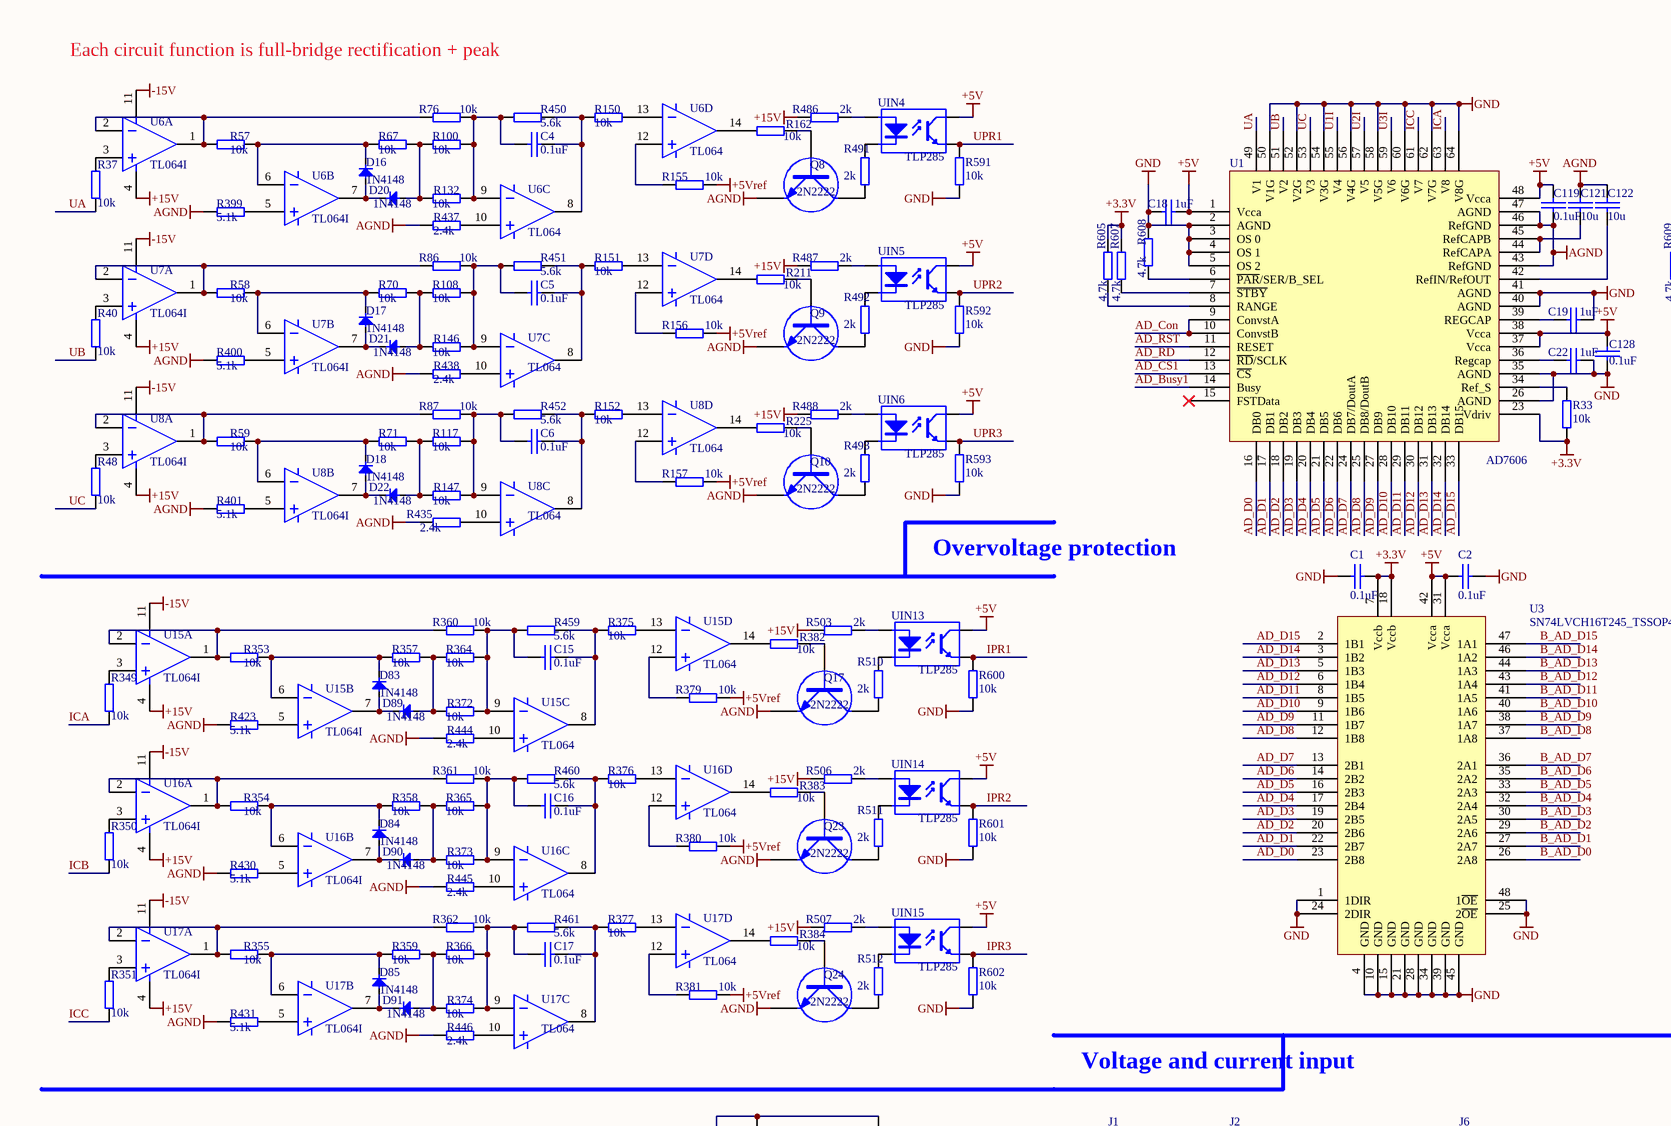
[diagram p0: MISC80584.SchDoc, top left]
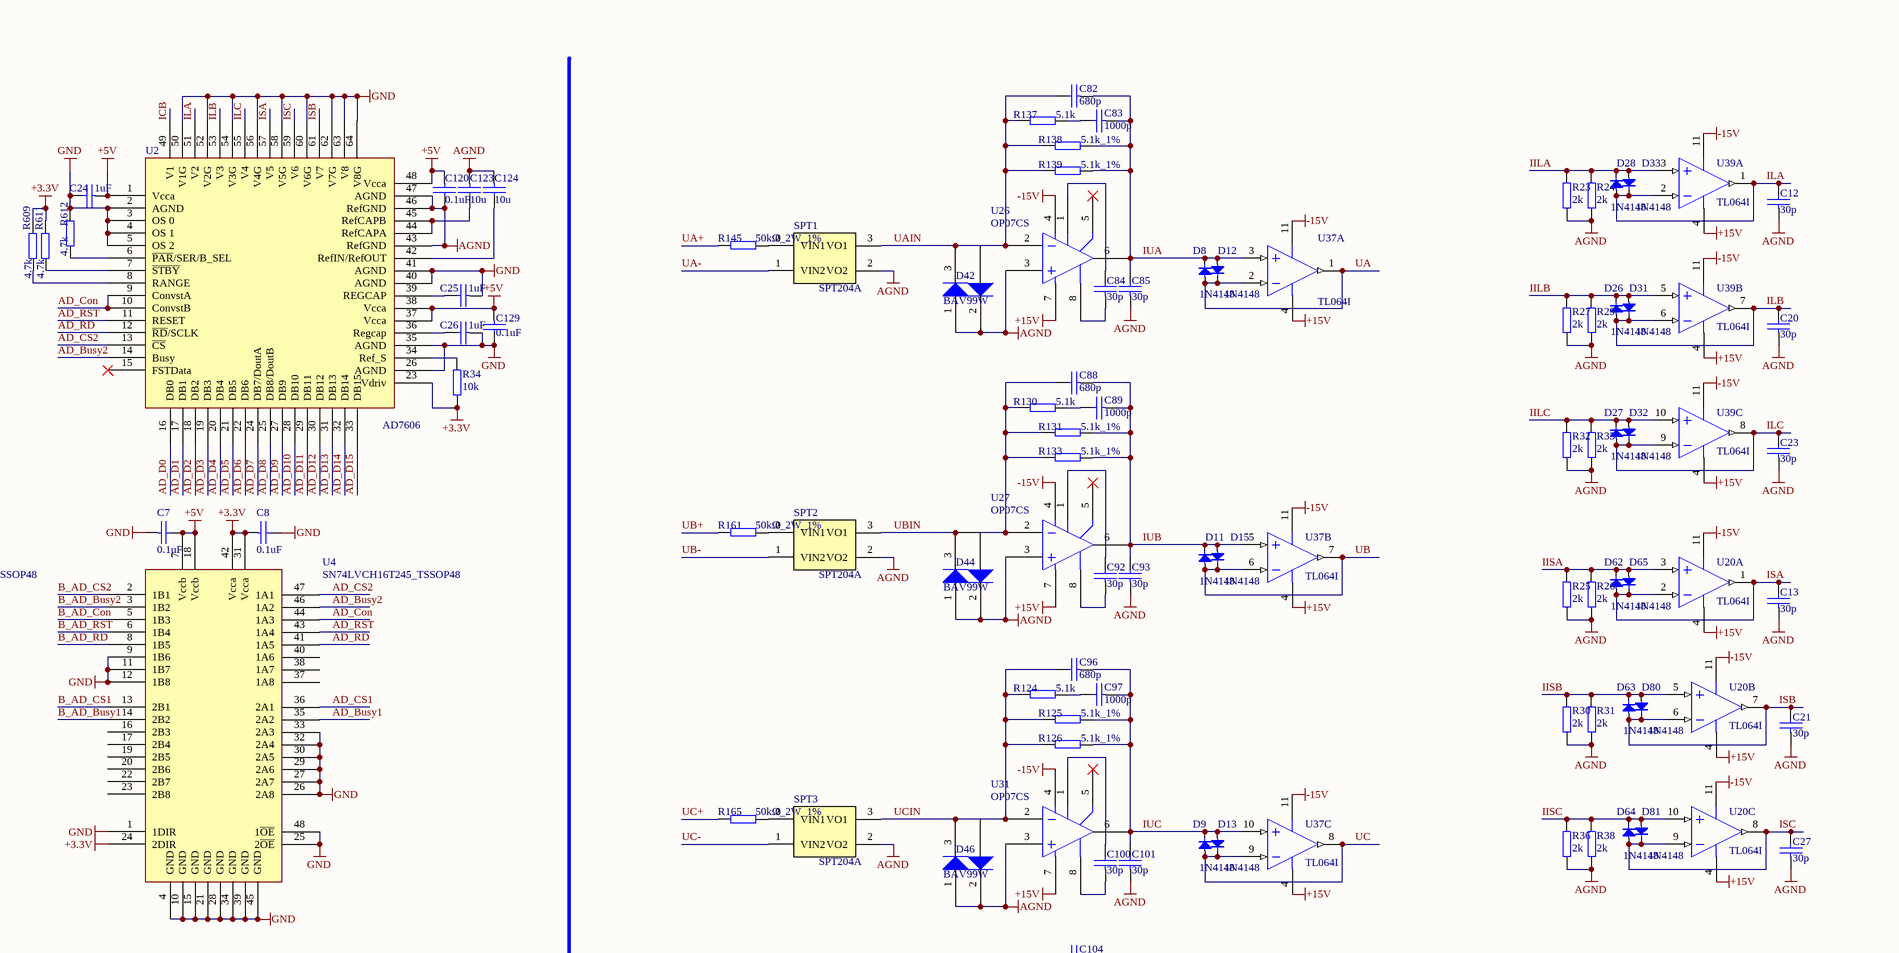
[diagram p1: MISC80584.SchDoc, top right]
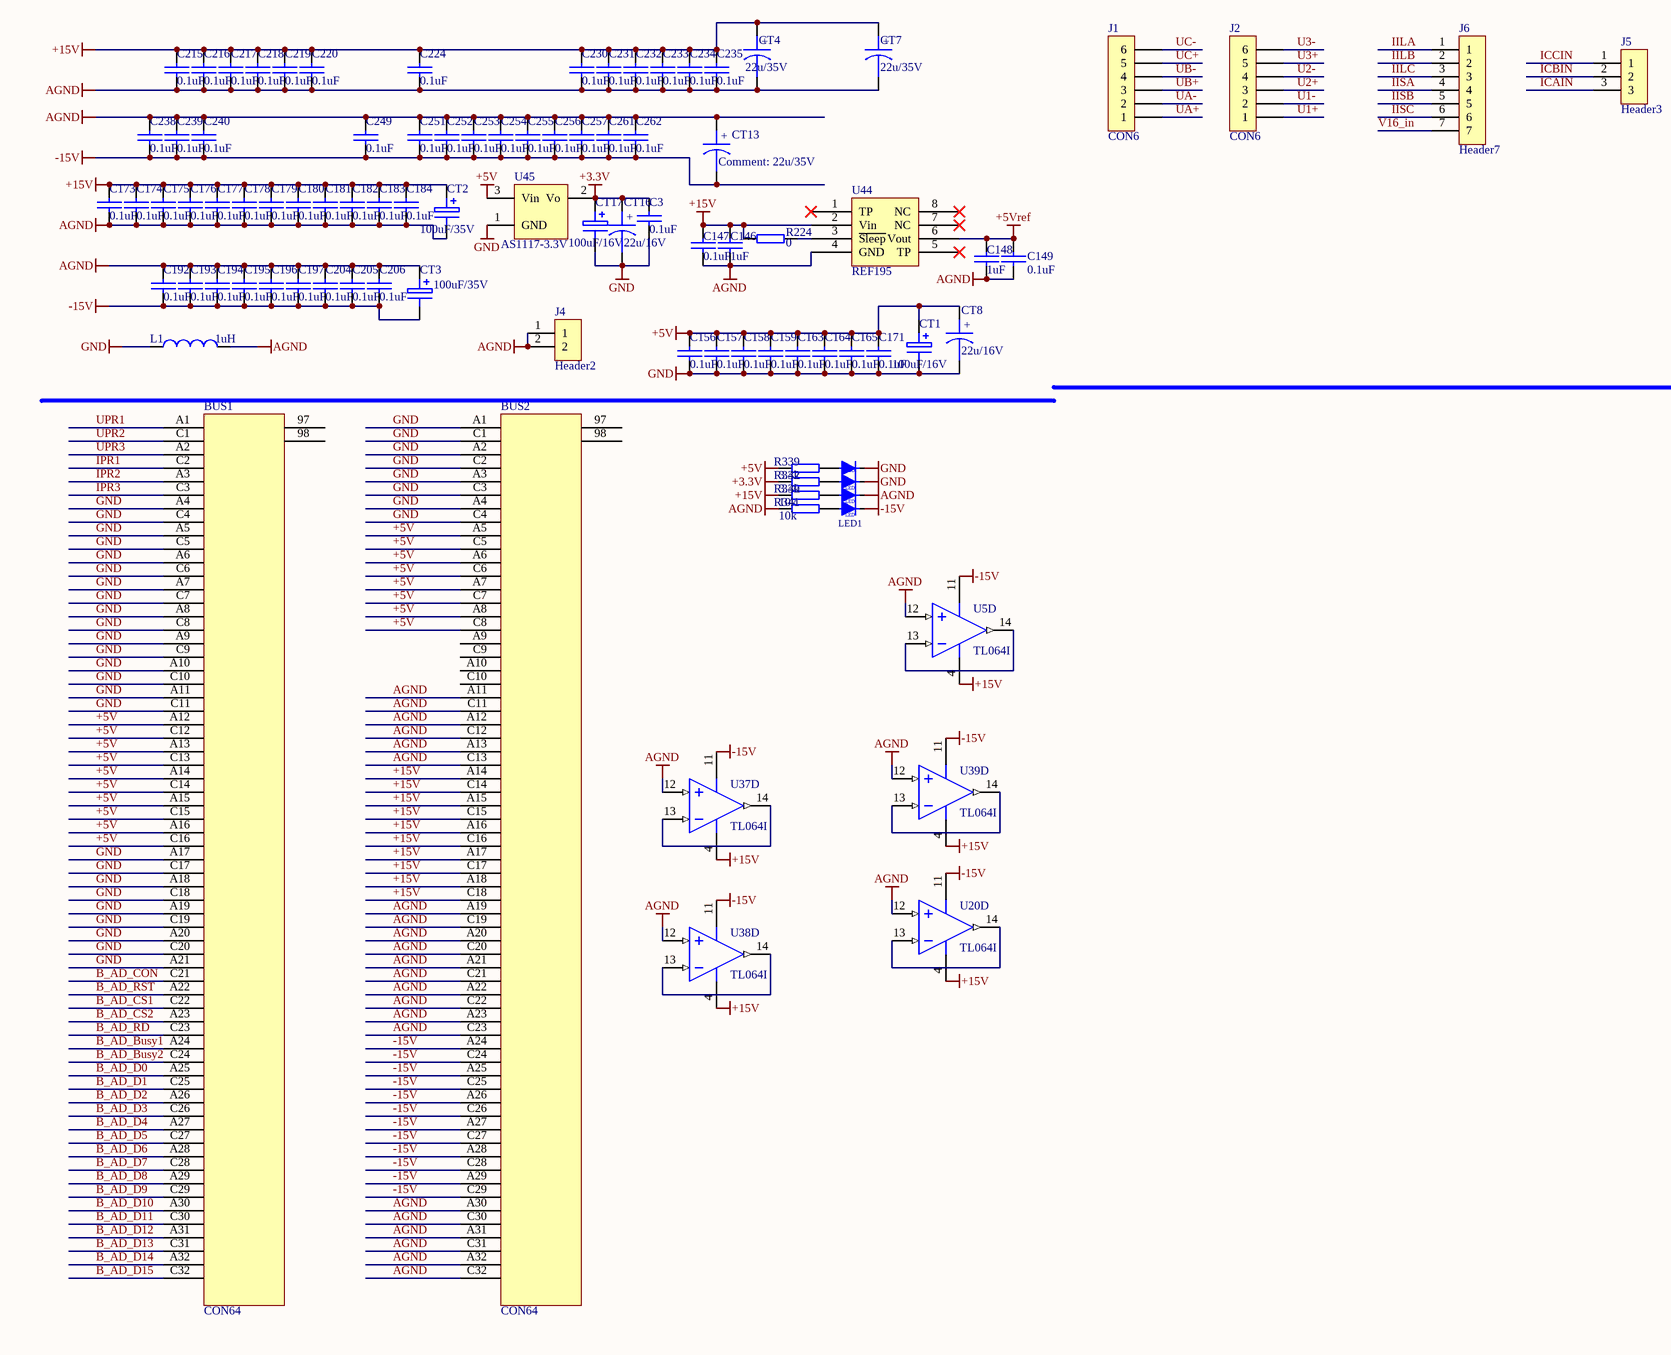
[diagram p2: MISC80584.SchDoc, bottom left]
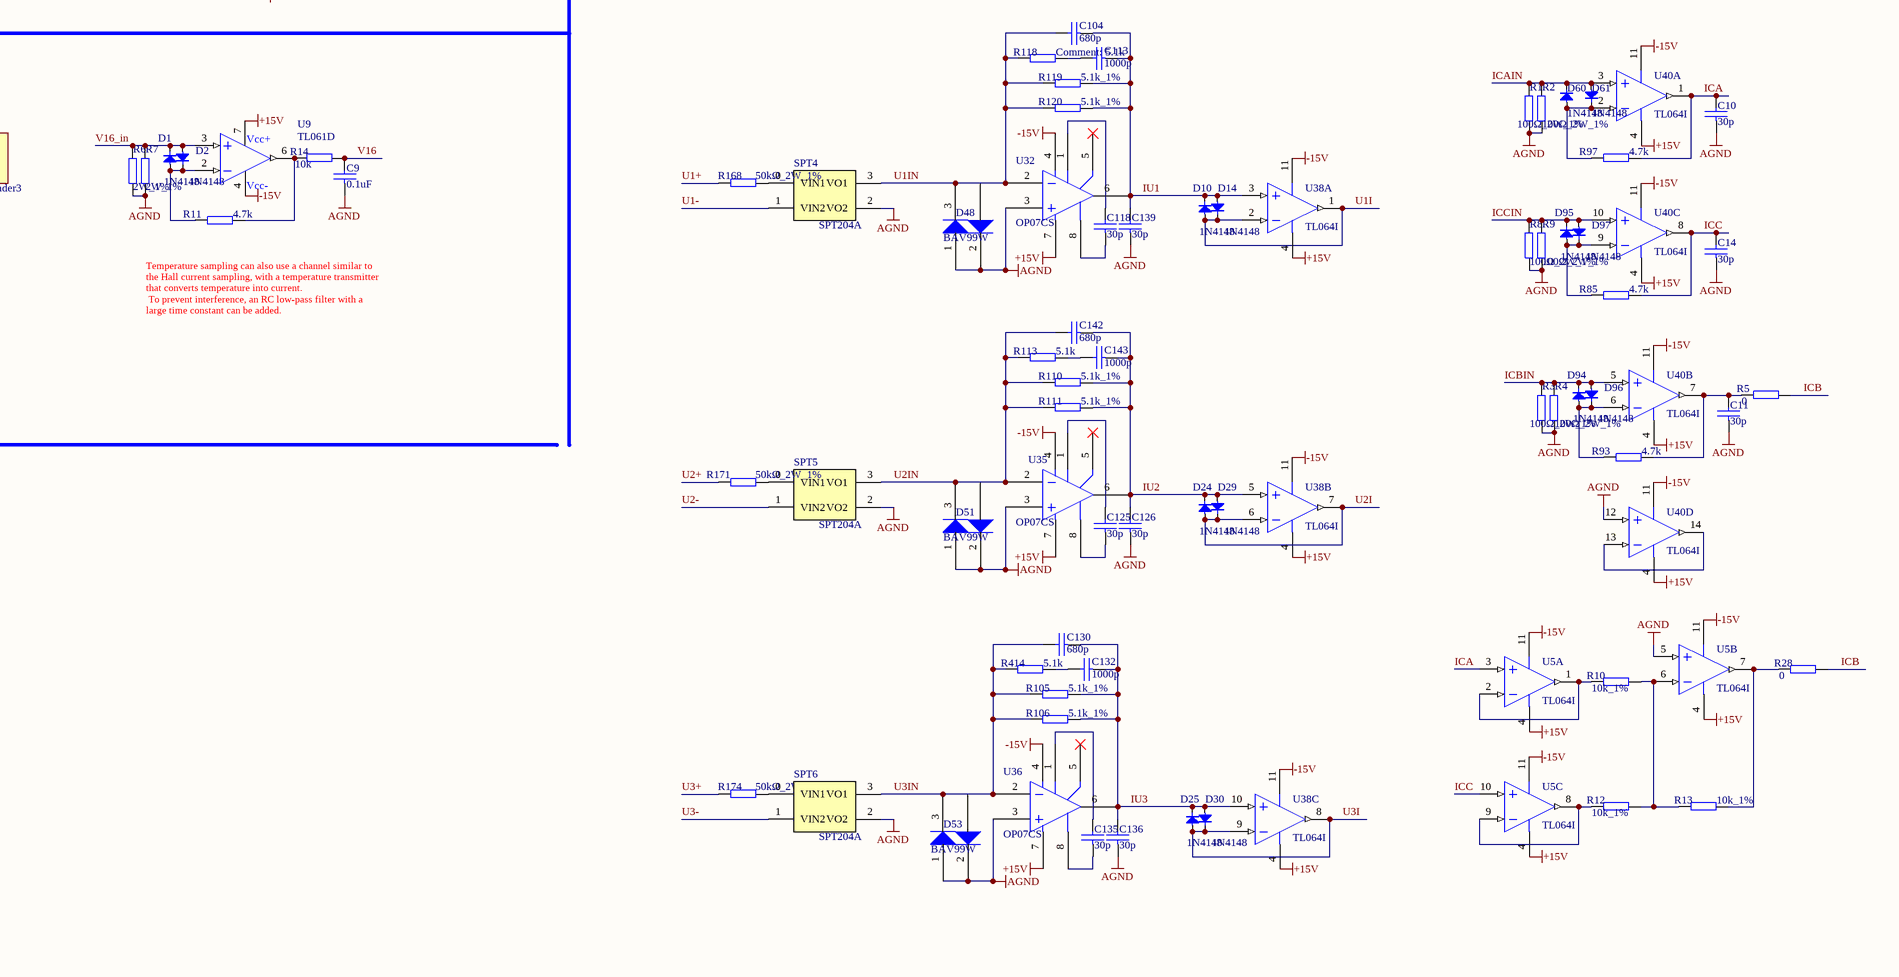
[diagram p3: MISC80584.SchDoc, bottom right]
# Altium project MISC80584.PrjPCB
1 sheet, 386 parts. Net scope: global (net labels, ports and power ports of the same name join across sheets).
Board file: MISC80584.PCBDoc

## Sheet MISC80584.SchDoc
size 762 x 457 mm; SheetNumber: 0; SheetTotal: 0

### Parts
BUS1  CON64  [BUS64W-A]
BUS2  CON64  [BUS64W-A]
C1  0.1uF  [0603]
C2  0.1uF  [0603]
C3  0.1uF  [0603]
C4  0.1uF  [0603]
C5  0.1uF  [0603]
C6  0.1uF  [0603]
C7  0.1uF  [0603]
C8  0.1uF  [0603]
C9  0.1uF  [0603]
C10  30p  [0603]
C11  30p  [0603]
C12  30p  [0603]
C13  30p  [0603]
C14  30p  [0603]
C15  0.1uF  [0603]
C16  0.1uF  [0603]
C17  0.1uF  [0603]
C18  1uF  [0603]
C19  1uF  [0603]
C20  30p  [0603]
C21  30p  [0603]
C22  1uF  [0603]
C23  30p  [0603]
C24  1uF  [0603]
C25  1uF  [0603]
C26  1uF  [0603]
C27  30p  [0603]
C82  680p  [0603]
C83  1000p  [0603]
C84  30p  [0603]
C85  30p  [0603]
C88  680p  [0603]
C89  1000p  [0603]
C92  30p  [0603]
C93  30p  [0603]
C96  680p  [0603]
C97  1000p  [0603]
C100  30p  [0603]
C101  30p  [0603]
C104  680p  [0603]
C113  1000p  [0603]
C118  30p  [0603]
C119  0.1uF  [0603]
C120  0.1uF  [0603]
C121  10u  [0805]
C122  10u  [0805]
C123  10u  [0805]
C124  10u  [0805]
C125  30p  [0603]
C126  30p  [0603]
C128  0.1uF  [0603]
C129  0.1uF  [0603]
C130  680p  [0603]
C132  1000p  [0603]
C135  30p  [0603]
C136  30p  [0603]
C139  30p  [0603]
C142  680p  [0603]
C143  1000p  [0603]
C146  1uF  [0603]
C147  0.1uF  [0603]
C148  1uF  [0603]
C149  0.1uF  [0603]
C156  0.1uF  [0603]
C157  0.1uF  [0603]
C158  0.1uF  [0603]
C159  0.1uF  [0603]
C163  0.1uF  [0603]
C164  0.1uF  [0603]
C165  0.1uF  [0603]
C171  0.1uF  [0603]
C173  0.1uF  [0603]
C174  0.1uF  [0603]
C175  0.1uF  [0603]
C176  0.1uF  [0603]
C177  0.1uF  [0603]
C178  0.1uF  [0603]
C179  0.1uF  [0603]
C180  0.1uF  [0603]
C181  0.1uF  [0603]
C182  0.1uF  [0603]
C183  0.1uF  [0603]
C184  0.1uF  [0603]
C192  0.1uF  [0603]
C193  0.1uF  [0603]
C194  0.1uF  [0603]
C195  0.1uF  [0603]
C196  0.1uF  [0603]
C197  0.1uF  [0603]
C204  0.1uF  [0603]
C205  0.1uF  [0603]
C206  0.1uF  [0603]
C215  0.1uF  [0603]
C216  0.1uF  [0603]
C217  0.1uF  [0603]
C218  0.1uF  [0603]
C219  0.1uF  [0603]
C220  0.1uF  [0603]
C224  0.1uF  [0603]
C230  0.1uF  [0603]
C231  0.1uF  [0603]
C232  0.1uF  [0603]
C233  0.1uF  [0603]
C234  0.1uF  [0603]
C235  0.1uF  [0603]
C238  0.1uF  [0603]
C239  0.1uF  [0603]
C240  0.1uF  [0603]
C249  0.1uF  [0603]
C251  0.1uF  [0603]
C252  0.1uF  [0603]
C253  0.1uF  [0603]
C254  0.1uF  [0603]
C255  0.1uF  [0603]
C256  0.1uF  [0603]
C257  0.1uF  [0603]
C261  0.1uF  [0603]
C262  0.1uF  [0603]
CT1  100uF/16V  [L470UF]
CT2  100uF/35V  [L470UF]
CT3  100uF/35V  [L470UF]
CT4  22u/35V  [7343_CASE-D]
CT7  22u/35V  [7343_CASE-D]
CT8  22u/16V  [3528_CASE-B]
CT13  22u/35V  [7343_CASE-D]
CT16  22u/16V  [3528_CASE-B]
CT17  100uF/16V  [L470UF]
D1  1N4148  [1N4148-A]
D2  1N4148  [1N4148-A]
D8  1N4148  [1N4148-A]
D9  1N4148  [1N4148-A]
D10  1N4148  [1N4148-A]
D11  1N4148  [1N4148-A]
D12  1N4148  [1N4148-A]
D13  1N4148  [1N4148-A]
D14  1N4148  [1N4148-A]
D15  1N4148  [1N4148-A]
D16  1N4148  [1N4148-A]
D17  1N4148  [1N4148-A]
D18  1N4148  [1N4148-A]
D20  1N4148  [1N4148-A]
D21  1N4148  [1N4148-A]
D22  1N4148  [1N4148-A]
D24  1N4148  [1N4148-A]
D25  1N4148  [1N4148-A]
D26  1N4148  [1N4148-A]
D27  1N4148  [1N4148-A]
D28  1N4148  [1N4148-A]
D29  1N4148  [1N4148-A]
D30  1N4148  [1N4148-A]
D31  1N4148  [1N4148-A]
D32  1N4148  [1N4148-A]
D33  1N4148  [1N4148-A]
D42  BAV99W  [SOT23R]
D44  BAV99W  [SOT23R]
D46  BAV99W  [SOT23R]
D48  BAV99W  [SOT23R]
D51  BAV99W  [SOT23R]
D53  BAV99W  [SOT23R]
D60  1N4148  [1N4148-A]
D61  1N4148  [1N4148-A]
D62  1N4148  [1N4148-A]
D63  1N4148  [1N4148-A]
D64  1N4148  [1N4148-A]
D65  1N4148  [1N4148-A]
D80  1N4148  [1N4148-A]
D81  1N4148  [1N4148-A]
D83  1N4148  [1N4148-A]
D84  1N4148  [1N4148-A]
D85  1N4148  [1N4148-A]
D89  1N4148  [1N4148-A]
D90  1N4148  [1N4148-A]
D91  1N4148  [1N4148-A]
D94  1N4148  [1N4148-A]
D95  1N4148  [1N4148-A]
D96  1N4148  [1N4148-A]
D97  1N4148  [1N4148-A]
J1  CON6  [EDGCon_6P_5.08mm_ear]
J2  CON6  [EDGCon_6P_5.08mm_ear]
J4  Header2  [EDGCON_2p_5.08mm_ear]
J5  Header3  [EDGCON_3p_5.08mm_ear]
J6  Header7  [EDGCon_7P_5.08mm_ear]
L1  1uH  [0805]
LED1  LEDGroup_4  [LEDGroup_4]  (value not drawn)
Q8  2N2222  [SOT23-3]
Q9  2N2222  [SOT23-3]
Q10  2N2222  [SOT23-3]
Q17  2N2222  [SOT23-3]
Q23  2N2222  [SOT23-3]
Q24  2N2222  [SOT23-3]
R1  100Ω_2W_1%  [AXIAL0.8]
R2  100Ω_2W_1%  [AXIAL0.8]
R3  100Ω_2W_1%  [AXIAL0.8]
R4  100Ω_2W_1%  [AXIAL0.8]
R5  0  [0603]
R6  2W_1%  [AXIAL0.8]
R7  2W_1%  [AXIAL0.8]
R8  100Ω_2W_1%  [AXIAL0.8]
R9  100Ω_2W_1%  [AXIAL0.8]
R10  10k_1%  [0603]
R11  4.7k  [0603]
R12  10k_1%  [0603]
R13  10k_1%  [0603]
R14  10k  [0603]
R23  2k  [0805]
R24  2k  [0805]
R25  2k  [0805]
R26  2k  [0805]
R27  2k  [0805]
R28  0  [0603]
R29  2k  [0805]
R30  2k  [0805]
R31  2k  [0805]
R32  2k  [0805]
R33  10k  [0603]
R34  10k  [0603]
R35  2k  [0805]
R36  2k  [0805]
R37  10k  [0603]
R38  2k  [0805]
R40  10k  [0603]
R48  10k  [0603]
R57  10k  [0603]
R58  10k  [0603]
R59  10k  [0603]
R67  10k  [0603]
R70  10k  [0603]
R71  10k  [0603]
R76  10k  [0603]
R85  4.7k  [0603]
R86  10k  [0603]
R87  10k  [0603]
R93  4.7k  [0603]
R97  4.7k  [0603]
R100  10k  [0603]
R105  5.1k_1%  [0603]
R106  5.1k_1%  [0603]
R108  10k  [0603]
R110  5.1k_1%  [0603]
R111  5.1k_1%  [0603]
R113  5.1k  [0603]
R117  10k  [0603]
R118  5.1k  [0603]
R119  5.1k_1%  [0603]
R120  5.1k_1%  [0603]
R124  5.1k  [0603]
R125  5.1k_1%  [0603]
R126  5.1k_1%  [0603]
R130  5.1k  [0603]
R131  5.1k_1%  [0603]
R132  10k  [0603]
R133  5.1k_1%  [0603]
R137  5.1k  [0603]
R138  5.1k_1%  [0603]
R139  5.1k_1%  [0603]
R145  50kΩ_2W_1%  [AXIAL0.8]
R146  10k  [0603]
R147  10k  [0603]
R150  10k  [0603]
R151  10k  [0603]
R152  10k  [0603]
R155  10k  [0603]
R156  10k  [0603]
R157  10k  [0603]
R161  50kΩ_2W_1%  [AXIAL0.8]
R162  10k  [0603]
R165  50kΩ_2W_1%  [AXIAL0.8]
R168  50kΩ_2W_1%  [AXIAL0.8]
R171  50kΩ_2W_1%  [AXIAL0.8]
R174  50kΩ_2W_1%  [AXIAL0.8]
R211  10k  [0603]
R224  0  [0603]
R225  10k  [0603]
R339  3.3k  [0603]
R340  10k  [0603]
R341  10k  [0603]
R342  3.3k  [0603]
R349  10k  [0603]
R350  10k  [0603]
R351  10k  [0603]
R353  10k  [0603]
R354  10k  [0603]
R355  10k  [0603]
R357  10k  [0603]
R358  10k  [0603]
R359  10k  [0603]
R360  10k  [0603]
R361  10k  [0603]
R362  10k  [0603]
R364  10k  [0603]
R365  10k  [0603]
R366  10k  [0603]
R372  10k  [0603]
R373  10k  [0603]
R374  10k  [0603]
R375  10k  [0603]
R376  10k  [0603]
R377  10k  [0603]
R379  10k  [0603]
R380  10k  [0603]
R381  10k  [0603]
R382  10k  [0603]
R383  10k  [0603]
R384  10k  [0603]
R399  5.1k  [0603]
R400  5.1k  [0603]
R401  5.1k  [0603]
R414  5.1k  [0603]
R423  5.1k  [0603]
R430  5.1k  [0603]
R431  5.1k  [0603]
R435  2.4k  [0603]
R437  2.4k  [0603]
R438  2.4k  [0603]
R444  2.4k  [0603]
R445  2.4k  [0603]
R446  2.4k  [0603]
R450  5.6k  [0603]
R451  5.6k  [0603]
R452  5.6k  [0603]
R459  5.6k  [0603]
R460  5.6k  [0603]
R461  5.6k  [0603]
R486  2k  [0603]
R487  2k  [0603]
R488  2k  [0603]
R491  2k  [0603]
R492  2k  [0603]
R493  2k  [0603]
R503  2k  [0603]
R506  2k  [0603]
R507  2k  [0603]
R510  2k  [0603]
R511  2k  [0603]
R512  2k  [0603]
R591  10k  [0603]
R592  10k  [0603]
R593  10k  [0603]
R600  10k  [0603]
R601  10k  [0603]
R602  10k  [0603]
R605  4.7k  [0603]
R607  4.7k  [0603]
R608  4.7k  [0603]
R609  4.7k  [0603]
R611  4.7k  [0603]
R612  4.7k  [0603]
SPT1  SPT204A  [SPT204A]
SPT2  SPT204A  [SPT204A]
SPT3  SPT204A  [SPT204A]
SPT4  SPT204A  [SPT204A]
SPT5  SPT204A  [SPT204A]
SPT6  SPT204A  [SPT204A]
U1  AD7606  [AD7606_LQFP64]
U2  AD7606  [AD7606_LQFP64]
U3  SN74LVCH16T245_TSSOP48  [SN74LVC16245_TSSOP48]
U4  SN74LVCH16T245_TSSOP48  [SN74LVC16245_TSSOP48]
U5  TL064I  [TL064D_SOIC-14]  (parts A,B,C,D of 4)
U6  TL064I  [TL064D_SOIC-14]  (parts A,B,C,D of 4)
U7  TL064I  [TL064D_SOIC-14]  (parts A,B,C,D of 4)
U8  TL064I  [TL064D_SOIC-14]  (parts A,B,C,D of 4)
U9  TL061D  [TL061_SOIC8]
U15  TL064I  [TL064D_SOIC-14]  (parts A,B,C,D of 4)
U16  TL064I  [TL064D_SOIC-14]  (parts A,B,C,D of 4)
U17  TL064I  [TL064D_SOIC-14]  (parts A,B,C,D of 4)
U20  TL064I  [TL064D_SOIC-14]  (parts A,B,C,D of 4)
U26  OP07CS  [SO-8]
U27  OP07CS  [SO-8]
U31  OP07CS  [SO-8]
U32  OP07CS  [SO-8]
U35  OP07CS  [SO-8]
U36  OP07CS  [SO-8]
U37  TL064I  [TL064D_SOIC-14]  (parts A,B,C,D of 4)
U38  TL064I  [TL064D_SOIC-14]  (parts A,B,C,D of 4)
U39  TL064I  [TL064D_SOIC-14]  (parts A,B,C,D of 4)
U40  TL064I  [TL064D_SOIC-14]  (parts A,B,C,D of 4)
U44  REF195  [SO-8]
U45  AS1117-3.3V  [SOT223]
UIN4  TLP285  [TLP285_SOP4]
UIN5  TLP285  [TLP285_SOP4]
UIN6  TLP285  [TLP285_SOP4]
UIN13  TLP285  [TLP285_SOP4]
UIN14  TLP285  [TLP285_SOP4]
UIN15  TLP285  [TLP285_SOP4]

### Nets
+3.3V: C1.2 C3.1 C8.1 CT16.1 CT17.1 R33.2 R34.2 R342.2 R605.2 R607.2 R609.2 R611.2 U1.23(Vdriv) U2.23(Vdriv) U3.7(Vccb) U3.18(Vccb) U4.24(2DIR) U4.31(Vcca) U4.42(Vcca) U45.2(Vo)
+5V: BUS1.A12 BUS1.A13 BUS1.A14 BUS1.A15 BUS1.A16 BUS1.C12 BUS1.C13 BUS1.C14 BUS1.C15 BUS1.C16 BUS2.A5 BUS2.A6 BUS2.A7 BUS2.A8 BUS2.C5 BUS2.C6 BUS2.C7 BUS2.C8 C2.1 C7.2 C18.1 C24.1 C119.1 C120.1 C128.1 C129.1 C156.2 C157.1 C158.1 C159.2 C163.1 C164.1 C165.2 C171.1 CT1.1 CT8.1 R339.2 U1.1(Vcca) U1.37(Vcca) U1.38(Vcca) U1.48(Vcca) U2.1(Vcca) U2.37(Vcca) U2.38(Vcca) U2.48(Vcca) U3.31(Vcca) U3.42(Vcca) U4.7(Vccb) U4.18(Vccb) U45.3(Vin) UIN4.4 UIN5.4 UIN6.4 UIN13.4 UIN14.4 UIN15.4
+5Vref: C148.1 C149.2 R155.2 R156.2 R157.2 R379.2 R380.2 R381.2 U44.6(Vout)
+15V: BUS2.A14 BUS2.A15 BUS2.A16 BUS2.A17 BUS2.A18 BUS2.C14 BUS2.C15 BUS2.C16 BUS2.C17 BUS2.C18 C146.1 C147.1 C173.2 C174.1 C175.1 C176.2 C177.1 C178.2 C179.2 C180.1 C181.1 C182.2 C183.2 C184.1 C215.1 C216.2 C217.2 C218.1 C219.2 C220.2 C224.1 C230.2 C231.1 C232.1 C233.2 C234.1 C235.2 CT2.1 CT4.1 CT7.1 R224.2 R340.2 R486.1 R487.1 R488.1 R503.1 R506.1 R507.1 U5.4(VCC) U6.4 U7.4 U8.4 U9.7(V+) U15.4 U16.4 U17.4 U20.4(VCC) U26.7 U27.7 U31.7 U32.7 U35.7 U36.7 U37.4(VCC) U38.4(VCC) U39.4(VCC) U40.4(VCC) U44.2(Vin)
-15V: BUS2.A24 BUS2.A25 BUS2.A26 BUS2.A27 BUS2.A28 BUS2.A29 BUS2.C24 BUS2.C25 BUS2.C26 BUS2.C27 BUS2.C28 BUS2.C29 C192.2 C193.1 C194.2 C195.1 C196.1 C197.2 C204.2 C205.2 C206.1 C238.2 C239.1 C240.1 C249.1 C251.2 C252.1 C253.2 C254.1 C255.1 C256.2 C257.2 C261.2 C262.1 CT3.2 CT13.2 LED1.8 U5.11(VEE) U6.11 U7.11 U8.11 U9.4(V-) U15.11 U16.11 U17.11 U20.11(VEE) U26.4 U27.4 U31.4 U32.4 U35.4 U36.4 U37.11(VEE) U38.11(VEE) U39.11(VEE) U40.11(VEE)
AGND: BUS2.A11 BUS2.A12 BUS2.A13 BUS2.A19 BUS2.A20 BUS2.A21 BUS2.A22 BUS2.A23 BUS2.A30 BUS2.A31 BUS2.A32 BUS2.C11 BUS2.C12 BUS2.C13 BUS2.C19 BUS2.C20 BUS2.C21 BUS2.C22 BUS2.C23 BUS2.C30 BUS2.C31 BUS2.C32 C9.1 C10.1 C11.1 C12.1 C13.1 C14.1 C20.1 C21.1 C23.1 C27.1 C85.1 C93.1 C101.1 C119.2 C120.2 C121.1 C122.1 C123.1 C124.1 C126.1 C136.1 C139.1 C146.2 C147.2 C148.2 C149.1 C173.1 C174.2 C175.2 C176.1 C177.2 C178.1 C179.1 C180.2 C181.2 C182.1 C183.1 C184.2 C192.1 C193.2 C194.1 C195.2 C196.2 C197.1 C204.1 C205.1 C206.2 C215.2 C216.1 C217.1 C218.2 C219.1 C220.1 C224.2 C230.1 C231.2 C232.2 C233.1 C234.2 C235.1 C238.1 C239.2 C240.2 C249.2 C251.1 C252.2 C253.1 C254.2 C255.2 C256.1 C257.1 C261.1 C262.2 CT2.2 CT3.1 CT4.2 CT7.2 CT13.1 D42.1 D42.2 D44.1 D44.2 D46.1 D46.2 D48.1 D48.2 D51.1 D51.2 D53.1 D53.2 J4.1 J4.2 L1.2 LED1.6 Q8.E Q9.E Q10.E Q17.E Q23.E Q24.E R1.1 R2.1 R3.1 R4.1 R6.1 R7.1 R8.1 R9.1 R23.2 R24.2 R25.2 R26.2 R27.2 R29.2 R30.2 R31.2 R32.2 R35.2 R36.2 R38.2 R341.2 R399.2 R400.2 R401.2 R423.2 R430.2 R431.2 R435.2 R437.2 R438.2 R444.2 R445.2 R446.2 SPT1.2(VO2) SPT2.2(VO2) SPT3.2(VO2) SPT4.2(VO2) SPT5.2(VO2) SPT6.2(VO2) U1.43(RefGND) U1.46(RefGND) U1.47(AGND) U2.43(RefGND) U2.46(RefGND) U2.47(AGND) U5.5(2_IN+) U5.12(4_IN+) U20.12(4_IN+) U26.3 U27.3 U31.3 U32.3 U35.3 U36.3 U37.12(4_IN+) U38.12(4_IN+) U39.12(4_IN+) U40.12(4_IN+) U44.4(GND)
GND: BUS1.A4 BUS1.A5 BUS1.A6 BUS1.A7 BUS1.A8 BUS1.A9 BUS1.A10 BUS1.A11 BUS1.A17 BUS1.A18 BUS1.A19 BUS1.A20 BUS1.A21 BUS1.C4 BUS1.C5 BUS1.C6 BUS1.C7 BUS1.C8 BUS1.C9 BUS1.C10 BUS1.C11 BUS1.C17 BUS1.C18 BUS1.C19 BUS1.C20 BUS2.A1 BUS2.A2 BUS2.A3 BUS2.A4 BUS2.C1 BUS2.C2 BUS2.C3 BUS2.C4 C1.1 C2.2 C3.2 C7.1 C8.2 C18.2 C19.1 C22.1 C24.2 C25.1 C26.1 C128.2 C129.2 C156.1 C157.2 C158.2 C159.1 C163.2 C164.2 C165.1 C171.2 CT1.2 CT8.2 CT16.2 CT17.2 L1.1 LED1.2 LED1.4 R591.1 R592.1 R593.1 R600.1 R601.1 R602.1 R608.2 R612.2 U1.2(AGND) U1.3(OS_0) U1.4(OS_1) U1.5(OS_2) U1.26(AGND) U1.35(AGND) U1.40(AGND) U1.41(AGND) U1.50(V1G) U1.52(V2G) U1.54(V3G) U1.56(V4G) U1.58(V5G) U1.60(V6G) U1.62(V7G) U1.64(V8G) U2.2(AGND) U2.3(OS_0) U2.4(OS_1) U2.5(OS_2) U2.26(AGND) U2.35(AGND) U2.40(AGND) U2.41(AGND) U2.50(V1G) U2.52(V2G) U2.54(V3G) U2.56(V4G) U2.58(V5G) U2.60(V6G) U2.62(V7G) U2.63(V8) U2.64(V8G) U3.1(1DIR) U3.4(GND) U3.10(GND) U3.15(GND) U3.21(GND) U3.24(2DIR) U3.25(2~{OE}) U3.28(GND) U3.34(GND) U3.39(GND) U3.45(GND) U3.48(1~{OE}) U4.1(1DIR) U4.4(GND) U4.9(1B6) U4.10(GND) U4.11(1B7) U4.12(1B8) U4.15(GND) U4.21(GND) U4.25(2~{OE}) U4.26(2A8) U4.27(2A7) U4.28(GND) U4.29(2A6) U4.30(2A5) U4.32(2A4) U4.33(2A3) U4.34(GND) U4.39(GND) U4.45(GND) U4.48(1~{OE}) U45.1(GND)
AD_Busy1: U1.14(Busy) U4.35(2A2)
AD_Busy2: U2.14(Busy) U4.46(1A2)
AD_Con: U1.9(ConvstA) U1.10(ConvstB) U2.9(ConvstA) U2.10(ConvstB) U4.44(1A3)
AD_CS1: U1.13(~{CS}) U4.36(2A1)
AD_CS2: U2.13(~{CS}) U4.47(1A1)
AD_D0: U1.16(DB0) U2.16(DB0) U3.23(2B8)
AD_D1: U1.17(DB1) U2.17(DB1) U3.22(2B7)
AD_D2: U1.18(DB2) U2.18(DB2) U3.20(2B6)
AD_D3: U1.19(DB3) U2.19(DB3) U3.19(2B5)
AD_D4: U1.20(DB4) U2.20(DB4) U3.17(2B4)
AD_D5: U1.21(DB5) U2.21(DB5) U3.16(2B3)
AD_D6: U1.22(DB6) U2.22(DB6) U3.14(2B2)
AD_D7: U1.24(DB7/DoutA) U2.24(DB7/DoutA) U3.13(2B1)
AD_D8: U1.25(DB8/DoutB) U2.25(DB8/DoutB) U3.12(1B8)
AD_D9: U1.27(DB9) U2.27(DB9) U3.11(1B7)
AD_D10: U1.28(DB10) U2.28(DB10) U3.9(1B6)
AD_D11: U1.29(DB11) U2.29(DB11) U3.8(1B5)
AD_D12: U1.30(DB12) U2.30(DB12) U3.6(1B4)
AD_D13: U1.31(DB13) U2.31(DB13) U3.5(1B3)
AD_D14: U1.32(DB14) U2.32(DB14) U3.3(1B2)
AD_D15: U1.33(DB15) U2.33(DB15) U3.2(1B1)
AD_RD: U1.12(~{RD}/SCLK) U2.12(~{RD}/SCLK) U4.41(1A5)
AD_RST: U1.11(RESET) U2.11(RESET) U4.43(1A4)
B_AD_Busy1: BUS1.A24 U4.14(2B2)
B_AD_Busy2: BUS1.C24 U4.3(1B2)
B_AD_CON: BUS1.C21 U4.5(1B3)
B_AD_CS1: BUS1.C22 U4.13(2B1)
B_AD_CS2: BUS1.A23 U4.2(1B1)
B_AD_D0: BUS1.A25 U3.26(2A8)
B_AD_D1: BUS1.C25 U3.27(2A7)
B_AD_D2: BUS1.A26 U3.29(2A6)
B_AD_D3: BUS1.C26 U3.30(2A5)
B_AD_D4: BUS1.A27 U3.32(2A4)
B_AD_D5: BUS1.C27 U3.33(2A3)
B_AD_D6: BUS1.A28 U3.35(2A2)
B_AD_D7: BUS1.C28 U3.36(2A1)
B_AD_D8: BUS1.A29 U3.37(1A8)
B_AD_D9: BUS1.C29 U3.38(1A7)
B_AD_D10: BUS1.A30 U3.40(1A6)
B_AD_D11: BUS1.C30 U3.41(1A5)
B_AD_D12: BUS1.A31 U3.43(1A4)
B_AD_D13: BUS1.C31 U3.44(1A3)
B_AD_D14: BUS1.A32 U3.46(1A2)
B_AD_D15: BUS1.C32 U3.47(1A1)
B_AD_RD: BUS1.C23 U4.8(1B5)
B_AD_RST: BUS1.A22 U4.6(1B4)
ICA: C10.2 R97.1 R349.2 U1.63(V8) U5.3(1_IN+) U40.1(1_OUT)
ICAIN: D60.K D61.A J5.3 R1.2 R2.2 U40.3(1_IN+)
ICB: R5.1 R28.1 R350.2 U2.49(V1)
ICBIN: D94.K D96.A J5.2 R3.2 R4.2 U40.5(2_IN+)
ICC: C14.2 R85.1 R351.2 U1.61(V7) U5.10(3_IN+) U40.8(3_OUT)
ICCIN: D95.K D97.A J5.1 R8.2 R9.2 U40.10(3_IN+)
IILA: D28.K D33.A J6.1 R23.1 R24.1 U39.3(1_IN+)
IILB: D26.K D31.A J6.2 R27.1 R29.1 U39.5(2_IN+)
IILC: D27.K D32.A J6.3 R32.1 R35.1 U39.10(3_IN+)
IISA: D62.K D65.A J6.4 R25.1 R26.1 U20.3(1_IN+)
IISB: D63.K D80.A J6.5 R30.1 R31.1 U20.5(2_IN+)
IISC: D64.K D81.A J6.6 R36.1 R38.1 U20.10(3_IN+)
ILA: C12.2 D28.A D33.K U2.51(V2) U39.1(1_OUT) U39.2(1_IN-)
ILB: C20.2 D26.A D31.K U2.53(V3) U39.6(2_IN-) U39.7(2_OUT)
ILC: C23.2 D27.A D32.K U2.55(V4) U39.8(3_OUT) U39.9(3_IN-)
IPR1: BUS1.C2 R600.2 UIN13.3
IPR2: BUS1.A3 R601.2 UIN14.3
IPR3: BUS1.C3 R602.2 UIN15.3
ISA: C13.2 D62.A D65.K U2.57(V5) U20.1(1_OUT) U20.2(1_IN-)
ISB: C21.2 D63.A D80.K U2.61(V7) U20.6(2_IN-) U20.7(2_OUT)
ISC: C27.2 D64.A D81.K U2.59(V6) U20.8(3_OUT) U20.9(3_IN-)
IU1: C104.1 C113.1 C139.2 D10.K D14.A R119.1 R120.1 U32.6 U38.3(1_IN+)
IU2: C126.2 C142.1 C143.1 D24.K D29.A R110.1 R111.1 U35.6 U38.5(2_IN+)
IU3: C130.1 C132.1 C136.2 D25.K D30.A R105.1 R106.1 U36.6 U38.10(3_IN+)
IUA: C82.1 C83.1 C85.2 D8.K D12.A R138.1 R139.1 U26.6 U37.3(1_IN+)
IUB: C88.1 C89.1 C93.2 D11.K D15.A R131.1 R133.1 U27.6 U37.5(2_IN+)
IUC: C96.1 C97.1 C101.2 D9.K D13.A R125.1 R126.1 U31.6 U37.10(3_IN+)
U1+: J2.1 R168.2
U1-: J2.2 SPT4.1(VIN2)
U1I: D10.A D14.K U1.55(V4) U38.1(1_OUT) U38.2(1_IN-)
U1IN: C104.2 D48.3 R118.2 R119.2 R120.2 SPT4.3(VO1) U32.2
U2+: J2.3 R171.2
U2-: J2.4 SPT5.1(VIN2)
U2I: D24.A D29.K U1.57(V5) U38.6(2_IN-) U38.7(2_OUT)
U2IN: C142.2 D51.3 R110.2 R111.2 R113.2 SPT5.3(VO1) U35.2
U3+: J2.5 R174.2
U3-: J2.6 SPT6.1(VIN2)
U3I: D25.A D30.K U1.59(V6) U38.8(3_OUT) U38.9(3_IN-)
U3IN: C130.2 D53.3 R105.2 R106.2 R414.2 SPT6.3(VO1) U36.2
UA: D8.A D12.K R37.2 U1.49(V1) U37.1(1_OUT) U37.2(1_IN-)
UA+: J1.1 R145.2
UA-: J1.2 SPT1.1(VIN2)
UAIN: C82.2 D42.3 R137.2 R138.2 R139.2 SPT1.3(VO1) U26.2
UB: D11.A D15.K R40.2 U1.51(V2) U37.6(2_IN-) U37.7(2_OUT)
UB+: J1.3 R161.2
UB-: J1.4 SPT2.1(VIN2)
UBIN: C88.2 D44.3 R130.2 R131.2 R133.2 SPT2.3(VO1) U27.2
UC: D9.A D13.K R48.2 U1.53(V3) U37.8(3_OUT) U37.9(3_IN-)
UC+: J1.5 R165.2
UC-: J1.6 SPT3.1(VIN2)
UCIN: C96.2 D46.3 R124.2 R125.2 R126.2 SPT3.3(VO1) U31.2
UPR1: BUS1.A1 R591.2 UIN4.3
UPR2: BUS1.C1 R592.2 UIN5.3
UPR3: BUS1.A2 R593.2 UIN6.3
V16: C9.2 R14.1
V16_in: D1.K D2.A J6.7 R6.2 R7.2 U9.3(IN+)
NetC4_1: C4.1 R150.2 R450.1 U6.8
NetC4_2: C4.2 R76.1 R100.1 R132.1 R450.2 U6.9
NetC5_1: C5.1 R151.2 R451.1 U7.8
NetC5_2: C5.2 R86.1 R108.1 R146.1 R451.2 U7.9
NetC6_1: C6.1 R152.2 R452.1 U8.8
NetC6_2: C6.2 R87.1 R117.1 R147.1 R452.2 U8.9
NetC11_2: C11.2 R5.2 R93.1 U40.7(2_OUT)
NetC15_1: C15.1 R375.2 R459.1 U15.8
NetC15_2: C15.2 R360.1 R364.1 R372.1 R459.2 U15.9
NetC16_1: C16.1 R376.2 R460.1 U16.8
NetC16_2: C16.2 R361.1 R365.1 R373.1 R460.2 U16.9
NetC17_1: C17.1 R377.2 R461.1 U17.8
NetC17_2: C17.2 R362.1 R366.1 R374.1 R461.2 U17.9
NetC19_2: C19.2 U1.39(REGCAP)
NetC22_2: C22.2 U1.36(Regcap)
NetC25_2: C25.2 U2.39(REGCAP)
NetC26_2: C26.2 U2.36(Regcap)
NetC83_2: C83.2 R137.1
NetC84_1: C84.1 U26.8
NetC84_2: C84.2 U26.1
NetC89_2: C89.2 R130.1
NetC92_1: C92.1 U27.8
NetC92_2: C92.2 U27.1
NetC97_2: C97.2 R124.1
NetC100_1: C100.1 U31.8
NetC100_2: C100.2 U31.1
NetC113_2: C113.2 R118.1
NetC118_1: C118.1 U32.8
NetC118_2: C118.2 U32.1
NetC121_2: C121.2 U1.44(RefCAPA) U1.45(RefCAPB)
NetC122_2: C122.2 U1.42(RefIN/RefOUT)
NetC123_2: C123.2 U2.44(RefCAPA) U2.45(RefCAPB)
NetC124_2: C124.2 U2.42(RefIN/RefOUT)
NetC125_1: C125.1 U35.8
NetC125_2: C125.2 U35.1
NetC132_2: C132.2 R414.1
NetC135_1: C135.1 U36.8
NetC135_2: C135.2 U36.1
NetC143_2: C143.2 R113.1
NetD1_A: D1.A D2.K R11.2 U9.2(IN-)
NetD16_A: D16.A D20.K U6.7
NetD16_K: D16.K R57.1 R67.2 U6.6
NetD17_A: D17.A D21.K U7.7
NetD17_K: D17.K R58.1 R70.2 U7.6
NetD18_A: D18.A D22.K U8.7
NetD18_K: D18.K R59.1 R71.2 U8.6
NetD20_A: D20.A R67.1 R100.2 R132.2
NetD21_A: D21.A R70.1 R108.2 R146.2
NetD22_A: D22.A R71.1 R117.2 R147.2
NetD60_A: D60.A D61.K R97.2 U40.2(1_IN-)
NetD83_A: D83.A D89.K U15.7
NetD83_K: D83.K R353.1 R357.2 U15.6
NetD84_A: D84.A D90.K U16.7
NetD84_K: D84.K R354.1 R358.2 U16.6
NetD85_A: D85.A D91.K U17.7
NetD85_K: D85.K R355.1 R359.2 U17.6
NetD89_A: D89.A R357.1 R364.2 R372.2
NetD90_A: D90.A R358.1 R365.2 R373.2
NetD91_A: D91.A R359.1 R366.2 R374.2
NetD94_A: D94.A D96.K R93.2 U40.6(2_IN-)
NetD95_A: D95.A D97.K R85.2 U40.9(3_IN-)
NetLED1_1: LED1.1 R339.1
NetLED1_3: LED1.3 R342.1
NetLED1_5: LED1.5 R340.1
NetLED1_7: LED1.7 R341.1
NetQ8_B: Q8.B R162.1
NetQ8_C: Q8.C R491.2
NetQ9_B: Q9.B R211.1
NetQ9_C: Q9.C R492.2
NetQ10_B: Q10.B R225.1
NetQ10_C: Q10.C R493.2
NetQ17_B: Q17.B R382.1
NetQ17_C: Q17.C R510.2
NetQ23_B: Q23.B R383.1
NetQ23_C: Q23.C R511.2
NetQ24_B: Q24.B R384.1
NetQ24_C: Q24.C R512.2
NetR10_1: R10.1 R12.1 R13.2 U5.6(2_IN-)
NetR10_2: R10.2 U5.1(1_OUT) U5.2(1_IN-)
NetR11_1: R11.1 R14.2 U9.6(OUT)
NetR12_2: R12.2 U5.8(3_OUT) U5.9(3_IN-)
NetR13_1: R13.1 R28.2 U5.7(2_OUT)
NetR33_1: R33.1 U1.34(Ref_S)
NetR34_1: R34.1 U2.34(Ref_S)
NetR37_1: R37.1 U6.3
NetR40_1: R40.1 U7.3
NetR48_1: R48.1 U8.3
NetR57_2: R57.2 R76.2 U6.1 U6.2
NetR58_2: R58.2 R86.2 U7.1 U7.2
NetR59_2: R59.2 R87.2 U8.1 U8.2
NetR145_1: R145.1 SPT1.0(VIN1)
NetR150_1: R150.1 U6.13
NetR151_1: R151.1 U7.13
NetR152_1: R152.1 U8.13
NetR155_1: R155.1 U6.12
NetR156_1: R156.1 U7.12
NetR157_1: R157.1 U8.12
NetR161_1: R161.1 SPT2.0(VIN1)
NetR162_2: R162.2 U6.14
NetR165_1: R165.1 SPT3.0(VIN1)
NetR168_1: R168.1 SPT4.0(VIN1)
NetR171_1: R171.1 SPT5.0(VIN1)
NetR174_1: R174.1 SPT6.0(VIN1)
NetR211_2: R211.2 U7.14
NetR224_1: R224.1 U44.3(~{Sleep})
NetR225_2: R225.2 U8.14
NetR349_1: R349.1 U15.3
NetR350_1: R350.1 U16.3
NetR351_1: R351.1 U17.3
NetR353_2: R353.2 R360.2 U15.1 U15.2
NetR354_2: R354.2 R361.2 U16.1 U16.2
NetR355_2: R355.2 R362.2 U17.1 U17.2
NetR375_1: R375.1 U15.13
NetR376_1: R376.1 U16.13
NetR377_1: R377.1 U17.13
NetR379_1: R379.1 U15.12
NetR380_1: R380.1 U16.12
NetR381_1: R381.1 U17.12
NetR382_2: R382.2 U15.14
NetR383_2: R383.2 U16.14
NetR384_2: R384.2 U17.14
NetR399_1: R399.1 U6.5
NetR400_1: R400.1 U7.5
NetR401_1: R401.1 U8.5
NetR423_1: R423.1 U15.5
NetR430_1: R430.1 U16.5
NetR431_1: R431.1 U17.5
NetR435_1: R435.1 U8.10
NetR437_1: R437.1 U6.10
NetR438_1: R438.1 U7.10
NetR444_1: R444.1 U15.10
NetR445_1: R445.1 U16.10
NetR446_1: R446.1 U17.10
NetR486_2: R486.2 UIN4.1
NetR487_2: R487.2 UIN5.1
NetR488_2: R488.2 UIN6.1
NetR491_1: R491.1 UIN4.2
NetR492_1: R492.1 UIN5.2
NetR493_1: R493.1 UIN6.2
NetR503_2: R503.2 UIN13.1
NetR506_2: R506.2 UIN14.1
NetR507_2: R507.2 UIN15.1
NetR510_1: R510.1 UIN13.2
NetR511_1: R511.1 UIN14.2
NetR512_1: R512.1 UIN15.2
NetR605_1: R605.1 U1.8(RANGE)
NetR607_1: R607.1 U1.7(~{STBY})
NetR608_1: R608.1 U1.6(~{PAR}/SER/B_SEL)
NetR609_1: R609.1 U2.8(RANGE)
NetR611_1: R611.1 U2.7(~{STBY})
NetR612_1: R612.1 U2.6(~{PAR}/SER/B_SEL)
NetU5_13: U5.13(4_IN-) U5.14(4_OUT)
NetU20_13: U20.13(4_IN-) U20.14(4_OUT)
NetU37_13: U37.13(4_IN-) U37.14(4_OUT)
NetU38_13: U38.13(4_IN-) U38.14(4_OUT)
NetU39_13: U39.13(4_IN-) U39.14(4_OUT)
NetU40_13: U40.13(4_IN-) U40.14(4_OUT)

Not connected (* = marked no-connect by the designer): BUS1 97 98; BUS2 97 98 A9 A10 C9 C10; U1 15(FSTData)*; U2 15(FSTData)*; U4 16(2B3) 17(2B4) 19(2B5) 20(2B6) 22(2B7) 23(2B8) 37(1A8) 38(1A7) 40(1A6); U26 5*; U27 5*; U31 5*; U32 5*; U35 5*; U36 5*; U44 1(TP)* 5(TP)* 7(NC)* 8(NC)*

### Notes on the sheet
- Each circuit function is full-bridge rectification + peak comparison
  Taking channel U1 as an example, peak comparison voltage = U1*R450/R76
- Overvoltage protection
- Voltage and current input
- (near R11) Temperature sampling can also use a channel similar to the Hall current sampling, with a temperature transmitter that converts temperature into current.
  To prevent interference, an RC low-pass filter with a large time constant can be added.

### Library data of the parts
BUS1 BUS2 = CON64: Euro-style pin header, 64 positions
C1-C3 C7 C8 C18 C19 C22 C24-C26 C119-C124 C128 C129 C156-C159 C163-C165 C171 C173-C184 C192-C197 C204-C206 C215-C220 C224 C230-C235 C238-C240 C249 C251-C257 C261 C262 = CAP: Capacitor
C4-C6 C9-C17 C20 C21 C23 C27 C82-C85 C88 C89 C92 C93 C96 C97 C100 C101 C104 C113 C118 C125 C126 C130 C132 C135 C136 C139 C142 C143 C146-C149 = CAP
CT1-CT3 CT17 = EC
CT4 CT7 CT8 CT13 CT16 = CAPACITOR POL: Capacitor
D1 D2 D8-D18 D20-D22 D24-D33 D60-D65 D80 D81 D83-D85 D89-D91 D94-D97 = DIODE-S
D42 D44 D46 D48 D51 D53 = DDIODEB
J1 J2 = CON6: Connector
L1 = INDUCTOR
Q8-Q10 Q17 Q23 Q24 = NPN: NPN Transistor
R1-R14 R23-R38 R40 R48 R57-R59 R67 R70 R71 R76 R85-R87 R93 R97 R100 R105 R106 R108 R110 R111 R113 R117-R120 R124-R126 R130-R133 R137-R139 R145-R147 R150-R152 R155-R157 R161 R162 R165 R168 R171 R174 R211 R224 R225 R339-R342 R349-R351 R353-R355 R357-R362 R364-R366 R372-R377 R379-R384 R399-R401 R414 R423 R430 R431 R435 R437 R438 R444-R446 R450-R452 R459-R461 R486-R488 R491-R493 R503 R506 R507 R510-R512 R591-R593 R600-R602 R605 R607-R609 R611 R612 = RES2
SPT1-SPT6 = SPT
U3 U4 = SN74LVCH16T245: TI SN74LVCH16T245DGGR
U5 U20 U37-U40 = TL064I: Low Power Quad Operational Amplifier
U6-U8 U15-U17 = TL084
U26 U27 U31 U32 U35 U36 = LM101
U44 = REF195: U?
U45 = 7810
UIN4-UIN6 UIN13-UIN15 = 521-1: Optoisolator